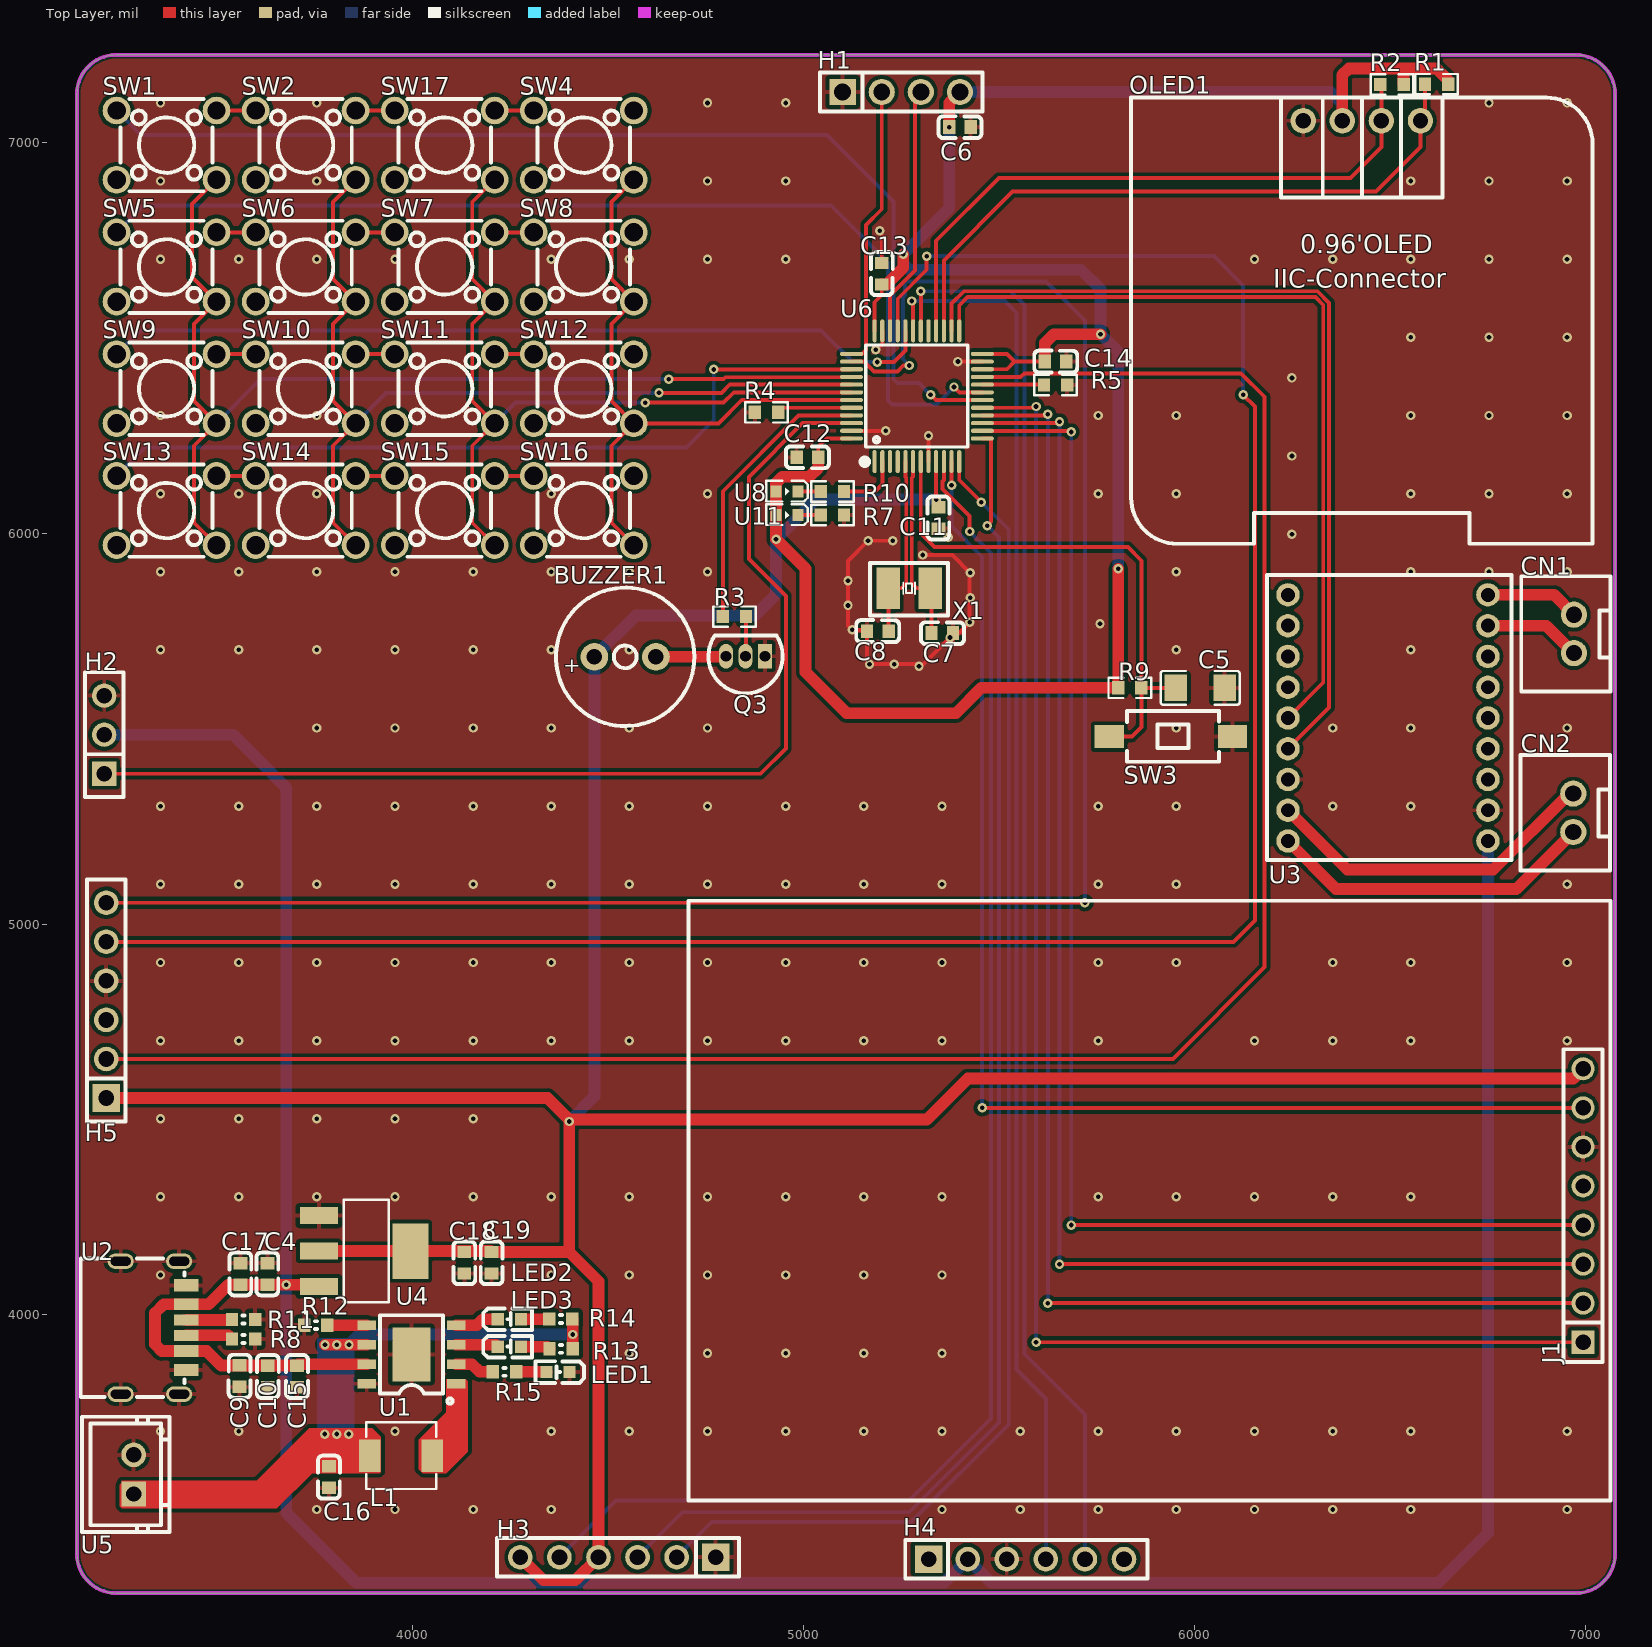
[diagram p0: Top Layer view]
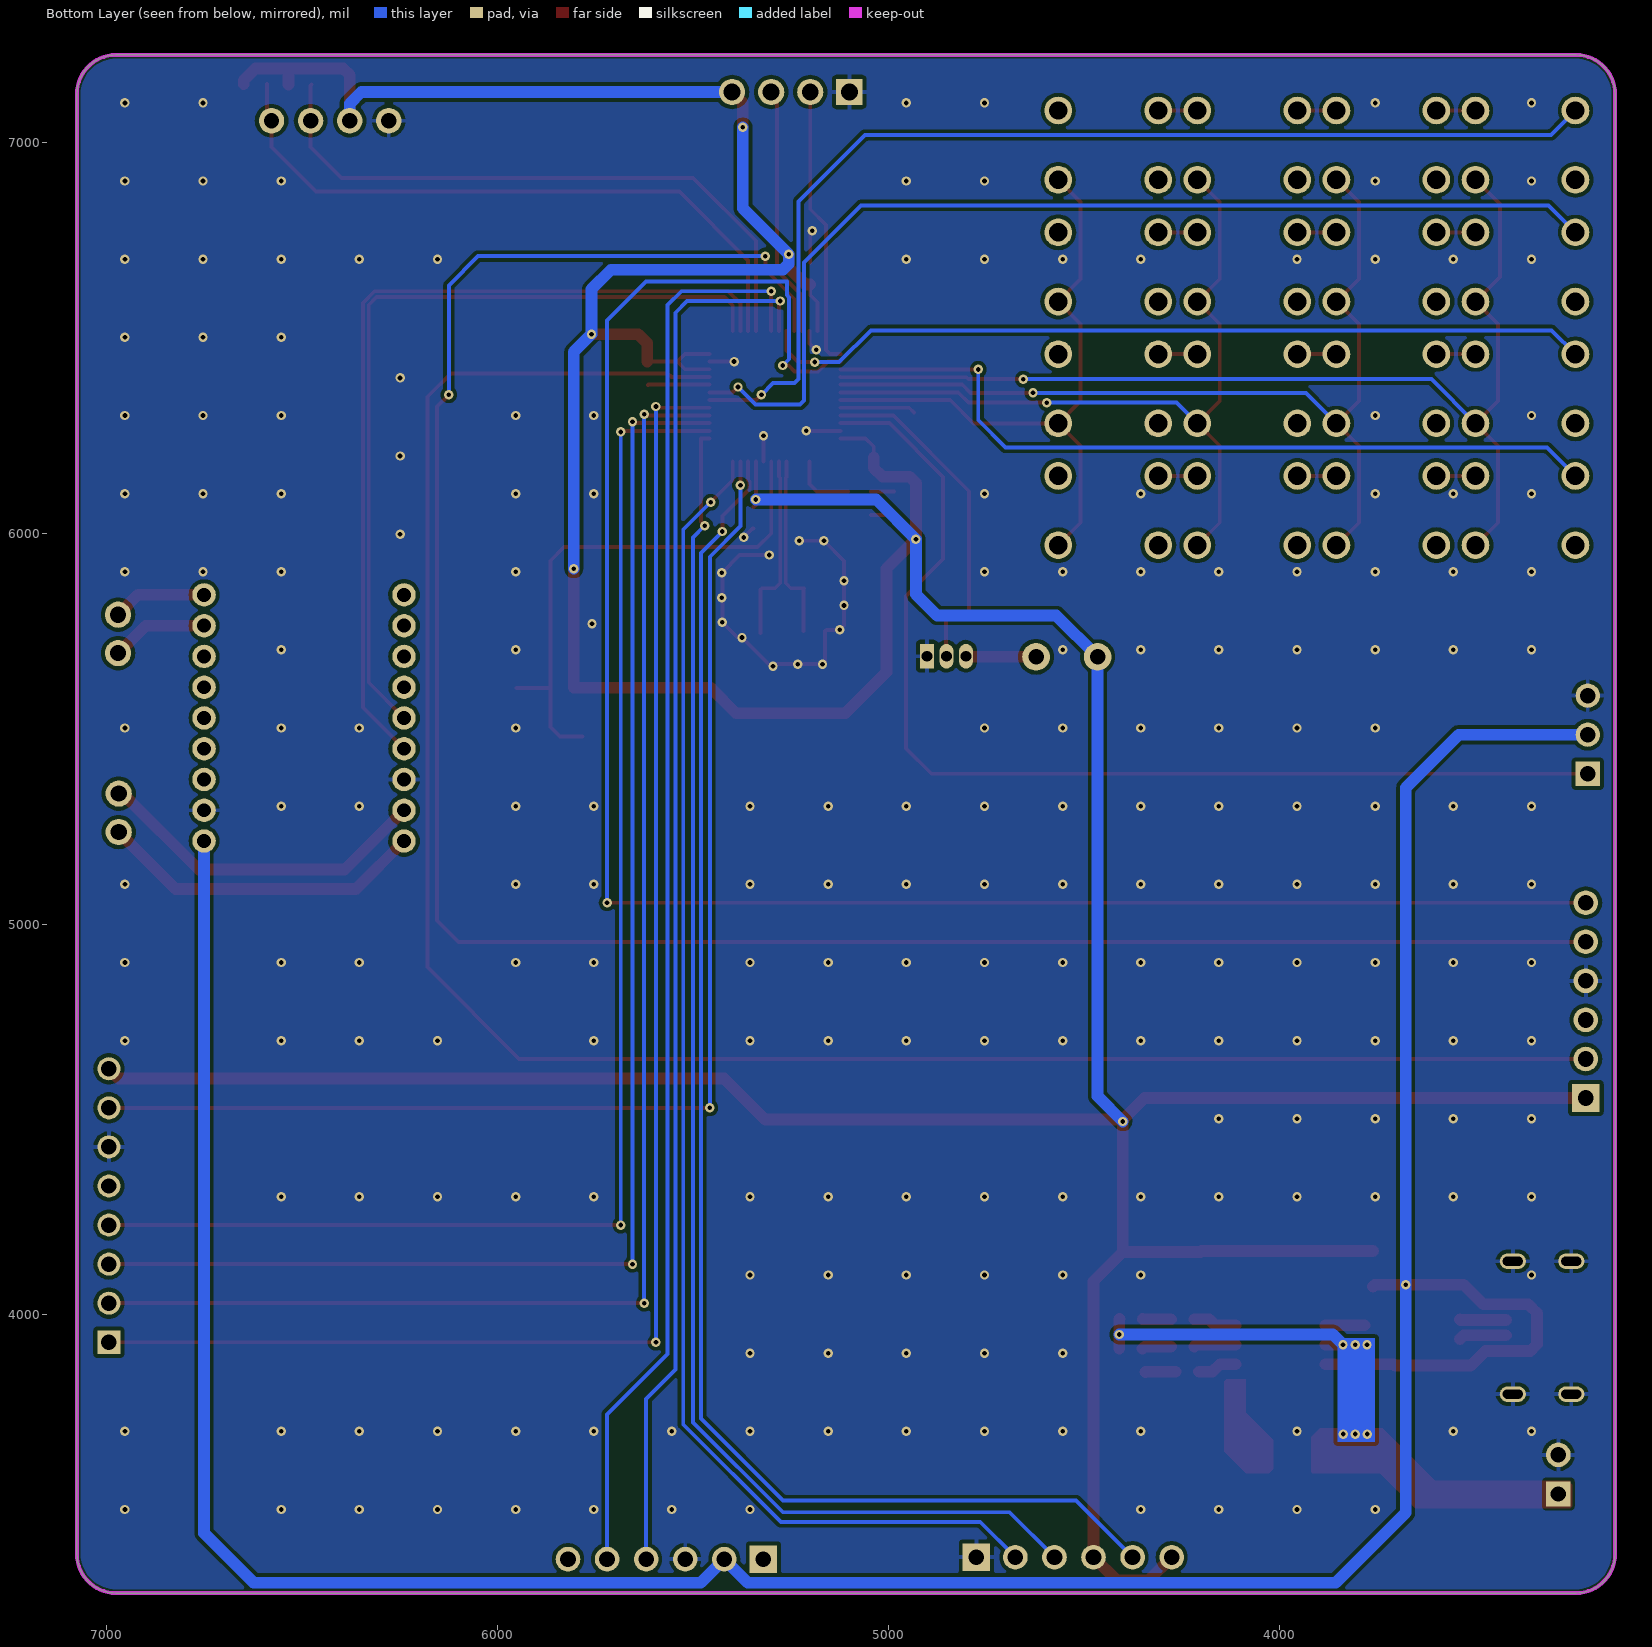
[diagram p1: Bottom Layer view, seen from below]
# Altium PCB MISC52129.pcbdoc
Units mil, origin at the board's own origin, x right, y up, seen from the top; angles counter-clockwise.
Board outline 3937.01 x 3937.01 mil, 2 copper layers (Top Layer, Bottom Layer), stack 62.206 mil thick; 71 components, 74 nets, 277 pads, 263 vias.

## Layer stack, top to bottom
Top Solder Mask Layer: solder mask 0.394, Dk 3.3
Top Layer: signal copper 1.379
Dielectric1: surface 59.449, FR4, Dk 4.5
Bottom Layer: signal copper 1.378
Bottom Solder Mask Layer: solder mask 0.394, Dk 3.3

## Board outline
3240,7225 ccw(c3240,7125) 3140,7125 3140,3387.99 ccw(c3240,3387.99) 3240,3287.99 6977.01,3287.99 ccw(c6977.01,3387.99) 7077.01,3387.99 7077.01,7125 ccw(c6977.01,7125) 6977.01,7225

## Design rules (kind name [scope] priority, off if disabled: settings)
BoardOutlineClearance copperThickness2oz_1 [All] p2 off: genericclearance=7.99 ignorepadtopadclearanceinfootprint=FALSE except(0: Arc-SplitContinuation Track-SplitContinuation SMDPad-SplitContinuation THPad-SplitContinuation Via-SplitContinuation Fill-SplitContinuation Region-SplitContinuation Poly-SplitContinuation Text-SplitContinuation Hole-SplitContinuation; 5.98: Arc-CutoutEdge Track-CutoutEdge SMDPad-CutoutEdge THPad-CutoutEdge Via-CutoutEdge Text-CutoutEdge; 6.9: Hole-OutlineEdge Hole-CutoutEdge; 10: Poly-OutlineEdge Poly-CutoutEdge; 11.81: Arc-OutlineEdge Track-OutlineEdge SMDPad-OutlineEdge THPad-OutlineEdge Via-OutlineEdge Fill-OutlineEdge Region-OutlineEdge Text-OutlineEdge Fill-CutoutEdge Region-CutoutEdge)
BoardOutlineClearance Plane_innerPlane_1 [All] p4 off: genericclearance=4.02 ignorepadtopadclearanceinfootprint=FALSE except(0: Arc-SplitContinuation Track-SplitContinuation SMDPad-SplitContinuation THPad-SplitContinuation Via-SplitContinuation Fill-SplitContinuation Region-SplitContinuation Poly-SplitContinuation Text-SplitContinuation Hole-SplitContinuation; 5.98: Arc-CutoutEdge Track-CutoutEdge SMDPad-CutoutEdge THPad-CutoutEdge Via-CutoutEdge Text-CutoutEdge; 6.9: Hole-OutlineEdge Hole-CutoutEdge; 10: Poly-OutlineEdge Poly-CutoutEdge; 11.81: Arc-OutlineEdge Track-OutlineEdge SMDPad-OutlineEdge THPad-OutlineEdge Via-OutlineEdge Fill-OutlineEdge Region-OutlineEdge Text-OutlineEdge Fill-CutoutEdge Region-CutoutEdge)
BoardOutlineClearance Copper_copperRegion_1 [All] p6 off: genericclearance=4.02 ignorepadtopadclearanceinfootprint=FALSE except(0: Arc-SplitContinuation Track-SplitContinuation SMDPad-SplitContinuation THPad-SplitContinuation Via-SplitContinuation Fill-SplitContinuation Region-SplitContinuation Poly-SplitContinuation Text-SplitContinuation Hole-SplitContinuation; 5.98: Arc-CutoutEdge Track-CutoutEdge SMDPad-CutoutEdge THPad-CutoutEdge Via-CutoutEdge Text-CutoutEdge; 6.9: Hole-OutlineEdge Hole-CutoutEdge; 10: Poly-OutlineEdge Poly-CutoutEdge; 11.81: Arc-OutlineEdge Track-OutlineEdge SMDPad-OutlineEdge THPad-OutlineEdge Via-OutlineEdge Fill-OutlineEdge Region-OutlineEdge Text-OutlineEdge Fill-CutoutEdge Region-CutoutEdge)
BoardOutlineClearance copperThickness1oz_1 [All] p8: genericclearance=4.02 ignorepadtopadclearanceinfootprint=FALSE except(0: Arc-SplitContinuation Track-SplitContinuation SMDPad-SplitContinuation THPad-SplitContinuation Via-SplitContinuation Fill-SplitContinuation Region-SplitContinuation Poly-SplitContinuation Text-SplitContinuation Hole-SplitContinuation; 5.98: Arc-CutoutEdge Track-CutoutEdge SMDPad-CutoutEdge THPad-CutoutEdge Via-CutoutEdge Text-CutoutEdge; 6.9: Hole-OutlineEdge Hole-CutoutEdge; 10: Poly-OutlineEdge Poly-CutoutEdge; 11.81: Arc-OutlineEdge Track-OutlineEdge SMDPad-OutlineEdge THPad-OutlineEdge Via-OutlineEdge Fill-OutlineEdge Region-OutlineEdge Text-OutlineEdge Fill-CutoutEdge Region-CutoutEdge)
Clearance copperThickness2oz [All] p1 off: gap=7.99 ignorepadtopadclearanceinfootprint=FALSE except(5.98: SMDPad-Track SMDPad-SMDPad THPad-Track SMDPad-THPad THPad-THPad Track-Via SMDPad-Via THPad-Via Via-Via Fill-SMDPad Region-SMDPad Fill-THPad Region-THPad Fill-Via Region-Via Fill-Fill Fill-Region Region-Region Arc-Track Arc-SMDPad Arc-THPad Arc-Via Fill-Arc Region-Arc Arc-Arc Text-Track SMDPad-Text Text-THPad Text-Via Fill-Text Region-Text Arc-Text Text-Text; 6.9: Hole-Track Hole-SMDPad Hole-THPad Hole-Via Fill-Hole Region-Hole Hole-Arc Hole-Text; 10: Poly-Track Poly-SMDPad Poly-THPad Poly-Via Poly-Fill Poly-Region Poly-Poly Poly-Arc Poly-Text Poly-Hole; 11.81: Fill-Track Region-Track)
Clearance Plane_innerPlane [All] p3 off: gap=4.02 ignorepadtopadclearanceinfootprint=FALSE except(5.98: SMDPad-Track SMDPad-SMDPad THPad-Track SMDPad-THPad THPad-THPad Track-Via SMDPad-Via THPad-Via Via-Via Fill-SMDPad Region-SMDPad Fill-THPad Region-THPad Fill-Via Region-Via Fill-Fill Fill-Region Region-Region Arc-Track Arc-SMDPad Arc-THPad Arc-Via Fill-Arc Region-Arc Arc-Arc Text-Track SMDPad-Text Text-THPad Text-Via Fill-Text Region-Text Arc-Text Text-Text; 6.9: Hole-Track Hole-SMDPad Hole-THPad Hole-Via Fill-Hole Region-Hole Hole-Arc Hole-Text; 10: Poly-Track Poly-SMDPad Poly-THPad Poly-Via Poly-Fill Poly-Region Poly-Poly Poly-Arc Poly-Text Poly-Hole; 11.81: Fill-Track Region-Track)
Clearance Copper_copperRegion [All] p5 off: gap=4.02 ignorepadtopadclearanceinfootprint=FALSE except(5.98: SMDPad-Track SMDPad-SMDPad THPad-Track SMDPad-THPad THPad-THPad Track-Via SMDPad-Via THPad-Via Via-Via Fill-SMDPad Region-SMDPad Fill-THPad Region-THPad Fill-Via Region-Via Fill-Fill Fill-Region Region-Region Arc-Track Arc-SMDPad Arc-THPad Arc-Via Fill-Arc Region-Arc Arc-Arc Text-Track SMDPad-Text Text-THPad Text-Via Fill-Text Region-Text Arc-Text Text-Text; 6.9: Hole-Track Hole-SMDPad Hole-THPad Hole-Via Fill-Hole Region-Hole Hole-Arc Hole-Text; 10: Poly-Track Poly-SMDPad Poly-THPad Poly-Via Poly-Fill Poly-Region Poly-Poly Poly-Arc Poly-Text Poly-Hole; 11.81: Fill-Track Region-Track)
Clearance copperThickness1oz [All] p7: gap=4.02 ignorepadtopadclearanceinfootprint=FALSE except(5.98: SMDPad-Track SMDPad-SMDPad THPad-Track SMDPad-THPad THPad-THPad Track-Via SMDPad-Via THPad-Via Via-Via Fill-SMDPad Region-SMDPad Fill-THPad Region-THPad Fill-Via Region-Via Fill-Fill Fill-Region Region-Region Arc-Track Arc-SMDPad Arc-THPad Arc-Via Fill-Arc Region-Arc Arc-Arc Text-Track SMDPad-Text Text-THPad Text-Via Fill-Text Region-Text Arc-Text Text-Text; 6.9: Hole-Track Hole-SMDPad Hole-THPad Hole-Via Fill-Hole Region-Hole Hole-Arc Hole-Text; 10: Poly-Track Poly-SMDPad Poly-THPad Poly-Via Poly-Fill Poly-Region Poly-Poly Poly-Arc Poly-Text Poly-Hole; 11.81: Fill-Track Region-Track)
DiffPairsRouting differentialPair [All] p1: maxlimit=6 minlimit=6 mostfreqgap=6 toplayer_minwidth=5 toplayer_prefwidth=10 toplayer_maxwidth=100 toplayer_mingap=6 toplayer_prefgap=6 toplayer_maxgap=6 bottomlayer_minwidth=5 bottomlayer_prefwidth=10 bottomlayer_maxwidth=100 bottomlayer_mingap=6 bottomlayer_prefgap=6 bottomlayer_maxgap=6 maxuncoupledlength=10
HoleToHoleClearance otherClearance [All] p1: gap=11.81 allowstackedmicrovias=TRUE
Length netLength [All] p1: minlimit=0 maxlimit=0
PasteMaskExpansion pasteMaskExpansion [All] p1: expansion=0
PlaneConnect innerPlane [All] p1: planeconnectstyle=Relief reliefexpansion=20 reliefentries=4 reliefconductorwidth=10 reliefairgap=10
PolygonConnect copperRegion [All] p1: connectstyle=Relief reliefconductorwidth=10 reliefentries=4 polygonreliefangle="90 Angle" airgapwidth=10 via.connectstyle=Relief via.reliefconductorwidth=10 via.reliefentries=4 via.polygonreliefangle="90 Angle" via.airgapwidth=10
RoutingVias viaSize [All] p1: holewidth=12.01 width=24.02 viastyle="Through Hole" minholewidth=11.81 minwidth=19.68 maxholewidth=248.03 maxwidth=393.7
SolderMaskExpansion solderMaskExpansion [IsVia] p1: expansion=-1000 istentingtop=TRUE
SolderMaskExpansion solderMaskExpansion [All] p2: expansion=2 istentingtop=FALSE
Width copperThickness2oz_2 [All] p1 off: maxlimit=100 minlimit=8 preferedwidth=10
Width copperThickness1oz_2 [All] p2: maxlimit=100 minlimit=5 preferedwidth=10

## Components (designator, comment, footprint, x,y, rotation, side; value= is the part's Value field where it differs from the comment)
BUZZER1 "2.7kHz" BUZ-TH_BD9.0-P4.00-D0.6-FD 4543.28,5684.32 r0 top
C4 "10uF" C0603 3627.51,4104.85 r270 top
C5 "100uF" C1206 6015,5605 r180 top
C6 "100nF" C0603 5400,7040 r180 top
C7 "20pF" C0603 5355,5745 r180 top
C8 "20pF" C0603 5190,5750 r0 top
C9 "22uF" C0603 3556.59,3843.41 r90 top
C10 "22uF" C0603 3628.64,3842.73 r90 top
C11 "100nF" C0603 5345,6040 r90 top
C12 "100nF" C0603 5010,6195 r0 top
C13 "100nF" C0603 5200,6665 r270 top
C14 "100nF" C0603 5645,6440 r180 top
C15 "22uF" C0603 3703.38,3842.73 r90 top
C16 "22uF" C0603 3785,3585 r90 top
C17 "100nF" C0603 3558.38,4104.85 r270 top
C18 "10uF" C0603 4131.59,4133.41 r90 top
C19 "100nF" C0603 4201.59,4133.41 r90 top
CN1 "XH2.54*2P_直插" CONN-TH_2P-P2.50-XH2.54-2P 6971.54,5742.95 r270 top
CN2 "XH2.54*2P_直插" CONN-TH_2P-P2.50-XH2.54-2P 6970,5285 r270 top
H1 "" HDR-TH_4P-P2.54-V-F 5250,7130 r0 top
H2 "" HDR-TH_3P-P2.54-V-F 3210,5485 r90 top
H3 "" HDR-TH_6P-P2.54-V-F 4525,3380 r180 top
H4 "" HDR-TH_6P-P2.54-V-F 5570,3375 r0 top
H5 "" HDR-TH_6P-P2.54-V-F 3215,4805 r90 top
J1 "" HDR-TH_8P-P2.54-V-M 6995,4280 r90 top
L1 "2.2uH" IND-SMD_L4.4-W4.2 3970,3640 r180 top
LED1 "电池" LED0603_L1.6-W0.8-RD_BLUE 4371.39,3853.75 r180 top
LED2 "放电" LED0603_L1.6-W0.8-RD_BLUE 4247.02,3988.81 r0 top
LED3 "充电" LED0603_L1.6-W0.8-RD_BLUE 4247.02,3918.81 r0 top
OLED1 "" 0.96OLED_4P 6428.8,7056.43 r0 top
Q3 "" S8050_TO_92 4851.43,5685.89 r180 top
R1 "5.1K" R0603 6620,7150 r0 top
R2 "5.1K" R0603 6505.98,7149.32 r0 top
R3 "1K" R0603 4822.85,5787.32 r180 top
R4 "10kΩ" R0603 4905,6310 r0 top
R5 "10kΩ" R0603 5645,6380 r180 top
R7 "510Ω" R0603 5073.8,6047.22 r0 top
R8 "5.1K" R0603-NSK 3566.59,3938.41 r180 top
R9 "1kΩ" R0603 5835,5605 r180 top
R10 "510Ω" R0603 5073.8,6107.52 r0 top
R11 "5.1K" R0603-NSK 3566.59,3988.41 r180 top
R12 "56K" R0603-NSK 3751.59,3973.91 r180 top
R13 "5.1K" R0603-NSK 4379.2,3913.13 r180 top
R14 "5.1K" R0603-NSK 4378.67,3989.49 r180 top
R15 "5.1K" R0603-NSK 4234.52,3854.37 r180 top
SW1 "KH-6X6X6H-TJ" SW-TH_4P-L6.0-W6.0-P4.50-LS6.5 3369.4,6994.04 r0 top
SW2 "KH-6X6X6H-TJ" SW-TH_4P-L6.0-W6.0-P4.50-LS6.5 3725.37,6994.04 r0 top
SW3 "TS-1101-C-W" SW-SMD_L6.0-W3.3-LS8.0 5940,5480 r180 top
SW4 "KH-6X6X6H-TJ" SW-TH_4P-L6.0-W6.0-P4.50-LS6.5 4437.3,6994.04 r0 top
SW5 "KH-6X6X6H-TJ" SW-TH_4P-L6.0-W6.0-P4.50-LS6.5 3369.4,6682.26 r0 top
SW6 "KH-6X6X6H-TJ" SW-TH_4P-L6.0-W6.0-P4.50-LS6.5 3725.37,6682.26 r0 top
SW7 "KH-6X6X6H-TJ" SW-TH_4P-L6.0-W6.0-P4.50-LS6.5 4081.33,6682.26 r0 top
SW8 "KH-6X6X6H-TJ" SW-TH_4P-L6.0-W6.0-P4.50-LS6.5 4437.3,6682.26 r0 top
SW9 "KH-6X6X6H-TJ" SW-TH_4P-L6.0-W6.0-P4.50-LS6.5 3369.4,6370.49 r0 top
SW10 "KH-6X6X6H-TJ" SW-TH_4P-L6.0-W6.0-P4.50-LS6.5 3725.37,6370.49 r0 top
SW11 "KH-6X6X6H-TJ" SW-TH_4P-L6.0-W6.0-P4.50-LS6.5 4081.33,6370.49 r0 top
SW12 "KH-6X6X6H-TJ" SW-TH_4P-L6.0-W6.0-P4.50-LS6.5 4437.3,6370.49 r0 top
SW13 "KH-6X6X6H-TJ" SW-TH_4P-L6.0-W6.0-P4.50-LS6.5 3369.4,6058.72 r0 top
SW14 "KH-6X6X6H-TJ" SW-TH_4P-L6.0-W6.0-P4.50-LS6.5 3725.37,6058.72 r0 top
SW15 "KH-6X6X6H-TJ" SW-TH_4P-L6.0-W6.0-P4.50-LS6.5 4081.33,6058.72 r0 top
SW16 "KH-6X6X6H-TJ" SW-TH_4P-L6.0-W6.0-P4.50-LS6.5 4437.3,6058.72 r0 top
SW17 "KH-6X6X6H-TJ" SW-TH_4P-L6.0-W6.0-P4.50-LS6.5 4081.33,6994.04 r0 top
U1 "ETA9742" ESOP-8_L4.9-W3.9-P1.27-LS6.0-BL-EP 3996.39,3898.81 r90 top
U2 "YTC-TC6-268" TYPE-C-SMD_YIYUAN_YTC-TC6-268 3335.87,3967.32 r270 top
U3 "CON2.0MM-PAD-18" CONN-TH_18P-P2.00_C9900078766 6751.54,5527.95 r90 top
U4 "AMS1117-3.3" SOT-223-3_L6.5-W3.4-P2.30-LS7.0-BR 3876.59,4163.41 r180 top
U5 "_x001F_XH2.54-2P" CONN-TH_2P-P2.54-V 3285.24,3591.72 r90 top
U6 "STM32F103C8T6" LQFP-48_L7.0-W7.0-P0.50-LS9.0-BL 5290.06,6351.43 r0 top
U8 "42-51/GHC-YW2X2K/3T" LED-SMD_L1.6-W0.8-FD_GREEN-1 4957.67,6107.52 r0 top
U11 "42-51/GHC-YW2X2K/3T" LED-SMD_L1.6-W0.8-FD_GREEN-1 4957.67,6047.22 r0 top
X1 "8MHz" CRYSTAL-SMD_L3.2-W2.5_3225-8MHZ 5270,5860 r180 top

## Footprints (in the part's own frame and the unit in brackets; to place one, negate y for a bottom-side part, rotate by r counter-clockwise, add the part's x,y. Pads: shape width x height; smd on the part's side, far side on the other; paste and mask are expansions set on the pad)
0.96OLED_4P [mm]
  round 1.65 hole 1 copper offset 0,0: 1(-3.81,-0.001) 2(-1.27,0.002) 3(1.27,0.002) 4(3.81,0.002)
  silkscreen extent -15,-27.5 15,1.5
BUZ-TH_BD9.0-P4.00-D0.6-FD [mm]
  round 1.8 hole 1: 1(-2,0) 2(2,0)
  silkscreen extent -4.5,-4.5 4.5,4.5
C0603 [mm]
  rect 0.8x0.9 smd: 1(-0.7,0) 2(0.7,0)
  silkscreen extent -1.39,-0.71 1.39,0.71
C1206 [mm]
  rect 1.485x1.728 smd paste-100 mask+0.051: 1(-1.593,0) 2(1.593,0)
  silkscreen extent -2.56,-1.09 2.56,1.09
CONN-TH_2P-P2.50-XH2.54-2P [mm]
  round 1.7 hole 1.05 paste+0 mask+0.05: 1(1.25,0) 2(-1.25,0)
  silkscreen extent -3.75,-3.42 3.75,2.37
CONN-TH_2P-P2.54-V [mm]
  rect 1.6x1.6 hole 1: 1(-1.27,0)
  round 1.6 hole 1: 2(1.27,0)
  silkscreen extent -3.75,-2.34 3.75,3.36
CONN-TH_18P-P2.00_C9900078766 [mil]
  round 60 hole 35.43 paste+0 mask+1.97: 1(-314.96,0.01) 2(-314.96,511.81) 3(-236.22,0.01) 4(-236.22,511.81) 5(-157.48,0.01) 6(-157.48,511.81) 9(0,0) 10(0,511.81) 11(78.74,0) 12(78.74,511.81) 13(157.48,0) 14(157.48,511.81) 15(236.22,0) 16(236.22,511.81) 17(314.96,0) 18(314.96,511.81)
  round 60 hole 35.43 copper offset -0.01,0 paste+0 mask+1.97: 7(-78.72,0.01) 8(-78.72,511.81)
  silkscreen extent -363,-60 365,565
CRYSTAL-SMD_L3.2-W2.5_3225-8MHZ [mil]
  rect 60x106.3 smd paste+0 mask+1.97: 1(-53.62,0) 2(53.62,0)
  silkscreen extent -100,-65 100,70
ESOP-8_L4.9-W3.9-P1.27-LS6.0-BL-EP [mm]
  rect 0.6x1.2 smd paste+0 mask+0.051: 1(-1.905,-2.908) 2(-0.635,-2.908) 3(0.635,-2.908) 4(1.905,-2.908) 5(1.905,2.908) 6(0.635,2.908) 7(-0.635,2.908) 8(-1.905,2.908)
  rect 3.5x2.5 smd paste+0 mask+0.051: 9(0,0)
  silkscreen extent -3.2,-2.67 2.55,2.05
HDR-TH_3P-P2.54-V-F [mil]
  rect 62x62 hole 40.16: 1(-100,0)
  round 62 hole 40.16: 2(0,0) 3(100,0)
  silkscreen extent -160,-49 160,49
HDR-TH_4P-P2.54-V-F [mm]
  rect 1.7x1.7 hole 1.1: 1(-3.81,0)
  round 1.7 hole 1.1: 2(-1.27,0) 3(1.27,0) 4(3.81,0)
  silkscreen extent -5.29,-1.27 5.29,1.27
HDR-TH_6P-P2.54-V-F [mm]
  rect 1.8x1.8 hole 1.02: 1(-6.35,0)
  round 1.6 hole 1.02: 2(-3.81,0) 3(-1.27,0) 4(1.27,0) 5(3.81,0) 6(6.35,0)
  silkscreen extent -7.87,-1.25 7.87,1.25
HDR-TH_8P-P2.54-V-M [mm]
  rect 1.5x1.5 hole 1: 1(-8.89,0)
  round 1.5 hole 1: 2(-6.35,0) 3(-3.81,0) 4(-1.27,0) 5(1.27,0) 6(3.81,0) 7(6.35,0) 8(8.89,0)
  silkscreen extent -10.16,-1.27 10.16,1.27
IND-SMD_L4.4-W4.2 [mm]
  rect 1.4x2.12 smd paste+0 mask+0.051: 1(2.028,0) 2(-2.028,0)
  silkscreen extent -2.28,-2.18 2.28,2.18
LED0603_L1.6-W0.8-RD_BLUE [mm]
  rect 0.8x0.8 smd: 1(-0.75,0) 2(0.75,0)
  silkscreen extent -1.7,-0.7 1.47,0.7
LED-SMD_L1.6-W0.8-FD_GREEN-1 [mm]
  rect 0.7x0.8 smd: 1(-0.715,0) 2(0.715,0)
  silkscreen extent -1.35,-0.65 1.35,0.7
LQFP-48_L7.0-W7.0-P0.50-LS9.0-BL [mm]
  oval 0.27x1.5 smd paste+0 mask+0.05: 1(-2.75,-4.25) 2(-2.25,-4.25) 3(-1.75,-4.25) 4(-1.25,-4.25) 5(-0.75,-4.25) 6(-0.25,-4.25) 7(0.25,-4.25) 8(0.75,-4.25) 9(1.25,-4.25) 10(1.75,-4.25) 11(2.25,-4.25) 12(2.75,-4.25) 25(2.75,4.25) 26(2.25,4.25) 27(1.75,4.25) 28(1.25,4.25) 29(0.75,4.25) 30(0.25,4.25) 31(-0.25,4.25) 32(-0.75,4.25) 33(-1.25,4.25) 34(-1.75,4.25) 35(-2.25,4.25) 36(-2.75,4.25)
  oval 1.5x0.27 smd paste+0 mask+0.05: 13(4.25,-2.75) 14(4.25,-2.25) 15(4.25,-1.75) 16(4.25,-1.25) 17(4.25,-0.75) 18(4.25,-0.25) 19(4.25,0.25) 20(4.25,0.75) 21(4.25,1.25) 22(4.25,1.75) 23(4.25,2.25) 24(4.25,2.75) 37(-4.25,2.75) 38(-4.25,2.25) 39(-4.25,1.75) 40(-4.25,1.25) 41(-4.25,0.75) 42(-4.25,0.25) 43(-4.25,-0.25) 44(-4.25,-0.75) 45(-4.25,-1.25) 46(-4.25,-1.75) 47(-4.25,-2.25) 48(-4.25,-2.75)
  silkscreen extent -3.59,-4.46 3.3,3.34
R0603 [mil]
  rect 31.75x34.02 smd paste-3937.01 mask+2: 1(-29.66,0) 2(29.66,0)
  silkscreen extent -55,-26 55,26
R0603-NSK [mil]
  rect 31.75x34.02 smd paste-3937.01 mask+2: 1(-29.65,0) 2(29.66,0)
  silkscreen extent -3,-10 3,10
S8050_TO_92 [mil]
  rect 35.4x63 hole 27.6 paste+0 mask+2: 1(-50,0)
  oval 35.4x63 hole 27.6 paste+0 mask+2: 2(0,0) 3(50,0)
  silkscreen extent -95,-53 95,95
SOT-223-3_L6.5-W3.4-P2.30-LS7.0-BR [mm]
  rect 2.5x1.1 smd: 1(2.97,-2.3) 2(2.97,0) 3(2.97,2.3)
  rect 2.34x3.6 smd: 4(-2.97,0)
  silkscreen extent -1.57,-3.33 1.37,3.33
SW-SMD_L6.0-W3.3-LS8.0 [mm]
  rect 1.9x1.5 smd: 1(-4,0) 2(4,0)
  silkscreen extent -3.14,-1.67 2.86,1.63
SW-TH_4P-L6.0-W6.0-P4.50-LS6.5 [mm]
  round 1.8 hole 1.2: 1(-3.25,2.25) 2(3.25,2.25) 3(-3.25,-2.25) 4(3.25,-2.25)
  silkscreen extent -3,-3 3,3
TYPE-C-SMD_YIYUAN_YTC-TC6-268 [mm]
  oval 1x1.7 hole 0.6 slot 1.3 at 90 deg paste+0 mask+0.05: 1(-4.32,1.676) 2(4.32,1.676) 3(4.32,-2.125) 4(-4.32,-2.125)
  rect 0.7x1.6 smd paste-100 mask+0.05: A5(-0.5,2.125) B5(0.5,2.125)
  rect 0.76x1.6 smd paste-100 mask+0.05: A9(1.52,2.125) B9(-1.52,2.125)
  rect 0.8x1.6 smd paste-100 mask+0.05: A12(2.75,2.125) B12(-2.75,2.125)
  silkscreen extent -4.5,-4.72 4.5,2.03

## Via types
v1: diameter 24.02, hole 12, Top Layer to Bottom Layer, 263 vias

## Nets (pads, with @x,y where several pads share a name; then routed paths per layer and width w, separated by ;. In a path a pad name is that pad's centre, name@x,y a point inside that pad or via, vN(x,y) a via of type N, cw(c..) or ccw(c..) an arc to the next point about the centre after c; other vN are vias at no path point)
$1N1877: BUZZER1.2 Q3.3 | length 180.1
  Top Layer w30: BUZZER1.2 4799.86,5684.32 Q3.3
$1N2018: Q3.2 R3.1 | length 101.9
  Top Layer w10: Q3.2 4852.51,5686.98 R3.1
$1N5108: R7.1 U11.2 | length 58.3
  Top Layer w10: U11.2 R7.1
$1N5109: R10.1 U8.2 | length 58.3
  Top Layer w10: U8.2 R10.1
$1N5277: SW9.2 SW10.1 | length 100.1
  Top Layer w10: SW9.2 SW10.1
$1N5278: SW13.2 SW14.1 | length 100.1
  Top Layer w10: SW13.2 SW14.1
$1N5279: SW15.2 SW16.1 | length 100.1
  Top Layer w10: SW15.2 SW16.1@4309.35,6147.3
$1N5280: SW14.2 SW15.1 | length 100.1
  Top Layer w10: SW14.2 SW15.1
$1N5281: SW11.2 SW12.1 | length 100.1
  Top Layer w10: SW11.2 SW12.1@4309.35,6459.07
$1N5282: SW10.2 SW11.1 | length 100.1
  Top Layer w10: SW10.2 SW11.1
$1N5283: SW7.2 SW8.1 | length 100.1
  Top Layer w10: SW7.2 SW8.1@4309.35,6770.84
$1N5284: SW5.2 SW6.1 | length 100.1
  Top Layer w10: SW5.2 SW6.1
$1N5285: SW6.2 SW7.1 | length 100.1
  Top Layer w10: SW6.2 SW7.1
$1N5286: SW1.2 SW2.1 | length 100.1
  Top Layer w10: SW1.2 SW2.1
$1N5287: SW2.2 SW17.1 | length 100.1
  Top Layer w10: SW2.2 SW17.1
$1N5288: SW4.1 SW17.2 | length 100.1
  Top Layer w10: SW17.2 SW4.1@4309.35,7082.62
$1N5308: LED3.2 R13.2 | length 75.3
  Top Layer w30: LED3.2 4343.87,3918.81 R13.2
$1N5310: LED1.2 R15.1 | length 77.9
  Top Layer w30: R15.1 4341.24,3854.37 LED1.2
$1N5311: LED2.2 R14.2 | length 72.8
  Top Layer w30: LED2.2 4348.33,3988.81 R14.2
$1N5312: LED2.1 U1.4 | length 112.8
  Top Layer w30: U1.4 4163.81,3973.81 4178.81,3988.81 LED2.1
$1N5313: R8.2 U2.B5 | length 121.2
  Top Layer w30: U2.B5 3527.72,3947.63 R8.2
$1N5314: R11.2 U2.A5 | length 118
  Top Layer w30: U2.A5 3535.52,3987 R11.2
$1N5317: LED3.1 U1.3 | length 108.7
  Top Layer w30: U1.3 4212.49,3923.81 LED3.1
$1N5319: R15.2 U1.2 | length 102
  Top Layer w30: U1.2 4151.19,3873.81 4170.63,3854.37 R15.2
$1N5320: R12.1 U1.5 | length 100.7
  Top Layer w30: R12.1 3881.79,3973.91 U1.5
$1N5322: L1.2 U1.1
+5V: C4.2 C9.2 C10.2 C15.2 C17.2 H2.2 H4.2 U1.7 U2.A9 U2.B9 U3.1 U4.3 | length 8498.4
  Top Layer w30: U4.3 3755.24,4077.29 v1(3676,4077.29) C4.2 C17.2 3527.29,4077.29 3477.16,4027.16 U2.B9 3362.16,4027.16 3340,4005 3340,3925 3357.53,3907.47 U2.A9 3472.53,3907.47 3509.71,3870.29 C10.2 C15.2 3706.9,3873.81 U1.7
  Bottom Layer w30: H2.2 3540,5485 3676,5349 v1(3676,4077.29) 3676,3494 3855.2,3314.8 5359.8,3314.8 5367.18,3322.18 ccw(c5355.43,3339.57) 5372.82,3327.82 H4.2 5480.2,3314.8 6624.8,3314.8 6751.53,3441.53 U3.1
BAT: C16.2 L1.1 R13.1 R14.1 U1.6 U5.1 | length 766.9
  Top Layer w30: v1(3775,3923.81) v1(3805.38,3923.81) v1(3836.32,3923.81) U1.6 ; R14.1 4408.85,3988.96 v1(4408.85,3950) R13.1
  Bottom Layer w30: v1(3836.32,3923.81) 3862.51,3950 v1(4408.85,3950)
  other v1: 3774.34,3695 3804.73,3695 3835.66,3695
BEEP: R3.2 U6.45 | length 730.8
  Top Layer w10: R3.2 4793.19,6108.19 4987.22,6302.22 U6.45
BOOT0: R4.2 U6.44 | length 193
  Top Layer w10: R4.2 4946.56,6321.9 U6.44
BOOT1: R5.2 U6.20 | length 158.4
  Top Layer w10: U6.20 5614.38,6380.96 R5.2
CLK: H1.2 U6.37 | length 718.1
  Top Layer w10: U6.37 5149.7,6459.7 5160,6470 5160,6790 5200,6830 H1.2
DIO: H1.3 U6.34 | length 643.9
  Top Layer w10: U6.34 5221.16,6609.6 5285,6673.44 5285,7115 H1.3
GND: C4.1 C5.1 C6.1 C7.1 C8.1 C9.1 C10.1 C11.1 C12.1 C13.1 C14.1 C15.1 C16.1 C17.1 C18.1 C19.1 H1.1 H2.3 H3.1 H4.3 H5.4 J1.6 LED1.1 OLED1.1 Q3.1 R4.1 R5.1 R7.2 R8.1 R11.1 R12.2 SW3.1 U1.8 U1.9 U2.1 U2.2 U2.3 U2.4 U2.A12 U2.B12 U3.3 U3.6 U4.1 U5.2 U6.8 U6.23 U6.35 U6.47 | length 1406.2
  Top Layer w10: U6.47 v1(5210,6262.85) ; v1(5185,6470) 5201.48,6486.48 U6.35 ; v1(5195,6775) 5200,6770 C13.1 ; v1(5228.39,5981.38) v1(5165,5981.38) 5113.62,5930 v1(5113.62,5879.29) v1(5113.62,5815.91) 5113.62,5764.28 v1(5124.45,5753.45) 5158.99,5753.45 C8.1 5162.44,5671.95 v1(5168.72,5665.67) v1(5232.1,5665.67) 5290.06,5665.67 v1(5295.27,5660.46) 5301.64,5660.46 v1(5374.81,5733.62) 5385.93,5733.62 v1(5424.84,5772.54) 5424.84,5897.75 v1(5426.38,5899.29) 5380.67,5945 v1(5305,5945) ; U6.8 v1(5319.59,6250) ; C11.1 5347.99,6012.44 v1(5370.44,5989.99) ; v1(5395,6440.01) U6.23
  other v1: 3754.1,3502.09 3954.1,3502.09 4154.1,3502.09 4354.1,3502.09 5354.1,3502.09 5554.1,3502.09 5754.1,3502.09 5954.1,3502.09 6154.1,3502.09 6354.1,3502.09 6554.1,3502.09 6954.1,3502.09 3354.1,3702.09 3554.1,3702.09 3954.1,3702.09 4354.1,3702.09 4554.1,3702.09 4754.1,3702.09 4954.1,3702.09 5154.1,3702.09 5354.1,3702.09 5554.1,3702.09 5754.1,3702.09 5954.1,3702.09 6154.1,3702.09 6354.1,3702.09 6554.1,3702.09 6954.1,3702.09 4554.1,3902.09 4754.1,3902.09 4954.1,3902.09 5154.1,3902.09 5354.1,3902.09 3354.1,4102.09 4354.1,4102.09 4554.1,4102.09 4754.1,4102.09 4954.1,4102.09 5154.1,4102.09 5354.1,4102.09 3354.1,4302.09 3554.1,4302.09 3754.1,4302.09 3954.1,4302.09 4154.1,4302.09 4354.1,4302.09 4554.1,4302.09 4754.1,4302.09 4954.1,4302.09 5154.1,4302.09 5354.1,4302.09 5754.1,4302.09 5954.1,4302.09 6154.1,4302.09 6354.1,4302.09 6554.1,4302.09 3354.1,4502.09 3554.1,4502.09 3754.1,4502.09 3954.1,4502.09 4154.1,4502.09 3354.1,4702.09 3554.1,4702.09 3754.1,4702.09 3954.1,4702.09 4154.1,4702.09 4354.1,4702.09 4554.1,4702.09 4754.1,4702.09 4954.1,4702.09 5154.1,4702.09 5354.1,4702.09 5754.1,4702.09 6154.1,4702.09 6354.1,4702.09 6554.1,4702.09 6954.1,4702.09 3354.1,4902.09 3554.1,4902.09 3754.1,4902.09 3954.1,4902.09 4154.1,4902.09 4354.1,4902.09 4554.1,4902.09 4754.1,4902.09 4954.1,4902.09 5154.1,4902.09 5354.1,4902.09 5754.1,4902.09 5954.1,4902.09 6354.1,4902.09 6554.1,4902.09 6954.1,4902.09 3354.1,5102.09 3554.1,5102.09 3754.1,5102.09 3954.1,5102.09 4154.1,5102.09 4354.1,5102.09 4554.1,5102.09 4754.1,5102.09 4954.1,5102.09 5154.1,5102.09 5354.1,5102.09 5754.1,5102.09 5954.1,5102.09 6954.1,5102.09 3354.1,5302.09 3554.1,5302.09 3754.1,5302.09 3954.1,5302.09 4154.1,5302.09 4354.1,5302.09 4554.1,5302.09 4754.1,5302.09 4954.1,5302.09 5154.1,5302.09 5354.1,5302.09 5754.1,5302.09 5954.1,5302.09 6354.1,5302.09 6554.1,5302.09 3754.1,5502.09 3954.1,5502.09 4154.1,5502.09 4354.1,5502.09 4554.1,5502.09 4754.1,5502.09 5954.1,5502.09 6354.1,5502.09 6554.1,5502.09 6954.1,5502.09 3354.1,5702.09 3554.1,5702.09 3754.1,5702.09 3954.1,5702.09 4154.1,5702.09 4354.1,5702.09 4554.1,5702.09 5954.1,5702.09 6554.1,5702.09 5758.62,5769.1 5426.38,5835.9 3354.1,5902.09 3554.1,5902.09 3754.1,5902.09 3954.1,5902.09 4154.1,5902.09 4354.1,5902.09 4554.1,5902.09 4754.1,5902.09 5954.1,5902.09 6554.1,5902.09 6754.1,5902.09 6954.1,5902.09 6249.78,5998.25 3354.1,6102.09 3554.1,6102.09 3754.1,6102.09 4354.1,6102.09 4754.1,6102.09 5754.1,6102.09 5954.1,6102.09 6554.1,6102.09 6754.1,6102.09 6954.1,6102.09 6249.78,6198.25 3354.1,6302.09 3754.1,6302.09 5754.1,6302.09 5954.1,6302.09 6554.1,6302.09 6754.1,6302.09 6954.1,6302.09 6249.78,6398.25 6554.1,6502.09 6754.1,6502.09 6954.1,6502.09 3354.1,6702.09 3554.1,6702.09 3754.1,6702.09 3954.1,6702.09 4354.1,6702.09 4554.1,6702.09 4754.1,6702.09 4954.1,6702.09 6154.1,6702.09 6354.1,6702.09 6554.1,6702.09 6754.1,6702.09 6954.1,6702.09 3354.1,6902.09 3754.1,6902.09 4754.1,6902.09 4954.1,6902.09 6554.1,6902.09 6754.1,6902.09 6954.1,6902.09 3354.1,7102.09 3754.1,7102.09 4754.1,7102.09 4954.1,7102.09 6754.1,7102.09 6954.1,7102.09
MFR_MISO: J1.4 U6.14 | length 3568.8
  Top Layer w10: U6.14 5682.15,6262.85 v1(5685,6260) ; v1(5685,4230) J1.4
  Bottom Layer w10: v1(5685,4230) v1(5685,6260)
MFR_MOSI: J1.3 U6.15 | length 3694.8
  Top Layer w10: U6.15 5651.69,6282.53 v1(5655,6285.84) ; v1(5655,4130) J1.3
  Bottom Layer w10: v1(5655,4130) v1(5655,6285.84)
MFR_RST: J1.7 U6.11 | length 3224.6
  Top Layer w10: U6.11 5378.64,6123.85 v1(5378.74,6123.74) ; v1(5457.01,4530) J1.7
  Bottom Layer w10: v1(5378.74,6123.74) 5378.74,6018.74 5457.01,5940.48 v1(5457.01,4530)
MFR_SCK: J1.2 U6.16 | length 3814.5
  Top Layer w10: U6.16 5621.7,6302.22 v1(5625,6305.52) ; v1(5625,4030) J1.2
  Bottom Layer w10: v1(5625,4030) v1(5625,6305.52)
MFR_SDA: J1.1 U6.17 | length 3934.2
  Top Layer w10: U6.17 5591.69,6321.9 v1(5595,6325.21) ; v1(5595,3930) J1.1
  Bottom Layer w10: v1(5595,3930) v1(5595,6325.21)
MIC+: CN1.1 U3.15 | length 249.2
  Top Layer w30: U3.15 6901.1,5764.17 CN1.1
MIC-: CN1.2 U3.17 | length 241
  Top Layer w30: U3.17 6920.79,5842.91 CN1.2
OLED_SCL: OLED1.3 R2.1 U6.28 | length 1630.8
  Top Layer w10: U6.28 5339.27,6749.27 5500,6910 6400,6910 6478.8,6988.8 OLED1.3 6478.8,7146.84 R2.1
OLED_SDA: OLED1.4 R1.1 U6.27 | length 1686.1
  Top Layer w10: U6.27 5358.96,6698.96 5535,6875 6465,6875 6578.8,6988.8 OLED1.4 6590.34,7068.02 R1.1
OSC32-IN: U6.3
OSC32-OUT: U6.4
OSC-IN: C8.2 U6.5 X1.2 | length 474.5
  Top Layer w10: C8.2 5217.56,5858.82 X1.2 5250,5860 5262.81,5872.81 5262.81,6142.19 5260.53,6144.47 U6.5
OSC-OUT: C7.2 U6.6 X1.1 | length 481.2
  Top Layer w10: U6.6 5280.22,6145.22 5276.82,6141.82 5276.82,5873.18 5290,5860 X1.1 5327.44,5856.18 C7.2
PA0: H3.5 U6.10 | length 3754
  Top Layer w10: U6.10 5358.96,6136.47 5355.75,6133.27 5355.75,6114.22 5425,6045 v1(5425,6005)
  Bottom Layer w10: H3.5 4520,3525 5270,3525 5480,3735 5480,5950 v1(5425,6005)
PA2: H3.2 U6.12 | length 3507.4
  Top Layer w10: U6.12 5398.33,6136.67 v1(5455,6080)
  Bottom Layer w10: H3.2 4765,3470 5275,3470 5525,3720 5525,6010 v1(5455,6080)
PA3: H3.3 U6.13 | length 3625.3
  Top Layer w10: U6.13 5480,6243.16 5480,6030 v1(5470,6020)
  Bottom Layer w10: H3.3 4690,3495 5270,3495 5500,3725 5500,5990 v1(5470,6020)
PA8: U6.29
PA9: H4.5 U6.30 | length 3655
  Top Layer w10: U6.30 5300,6518.86 v1(5300,6620)
  Bottom Layer w10: v1(5300,6620) 5530,6620 5565,6585 5565,3900 5720,3745 H4.5
PA10: H4.4 U6.31 | length 3579.1
  Top Layer w10: v1(5277.01,6595) 5280.22,6591.79 U6.31
  Bottom Layer w10: v1(5277.01,6595) 5515,6595 5545,6565 5545,3860 5620,3785 H4.4
PA11: SW9.1 U6.32 | length 2140.8
  Top Layer w10: v1(5188.79,6438.73) 5231.21,6438.73 5260.53,6468.04 U6.32
  Bottom Layer w10: SW9.1@3241.45,6459.07 3302.38,6520 5045,6520 5126.27,6438.73 v1(5188.79,6438.73)
PA12: H5.5 U6.33 | length 5663.2
  Top Layer w10: H5.5 6100,4955 6155,5010 6155,6325 v1(6125,6355) ; U6.33 5240.85,6600.85 5315,6675 v1(5315,6710)
  Bottom Layer w10: v1(5315,6710) 6050,6710 6125,6635 v1(6125,6355)
PA15: H5.6 U6.38 | length 4884.4
  Top Layer w10: H5.6 v1(5720,5055) ; U6.38 5154.99,6440.01 5180,6415 5240,6415 5255,6430 v1(5270,6430)
  Bottom Layer w10: v1(5270,6430) 5254.02,6445.98 5254.02,6604.52 5260,6610.51 5260,6645 5620,6645 5720,6545 v1(5720,5055)
PB0: SW1.1 U6.18 | length 2789.4
  Top Layer w10: v1(5325,6355) 5338.41,6341.59 U6.18
  Bottom Layer w10: SW1.1@3241.45,7082.62 3304.07,7020 5060,7020 5230,6850 5230,6395 5240,6385 5295,6385 v1(5325,6355)
PB1: SW5.1 U6.19 | length 2687.5
  Top Layer w10: v1(5385,6375) 5398.73,6361.27 U6.19
  Bottom Layer w10: SW5.1@3241.45,6770.84 3310.61,6840 5070,6840 5215.98,6694.02 5215.98,6340 5225.98,6330 5340,6330 v1(5385,6375)
PB3: SW13.1 U6.39 | length 2070.5
  Top Layer w10: v1(4770,6420) 5122.4,6420 U6.39
  Bottom Layer w10: SW13.1@3241.45,6147.3 3314.15,6220 4700,6220 4770,6290 v1(4770,6420)
PB4: SW1.4 SW5.4 SW9.4 SW13.4 U6.40 | length 2756.6
  Top Layer w10: SW13.4 3440,6027.49 3440,6224.56 SW9.4 3440,6339.26 3440,6536.33 SW5.4 3435,6656.03 3435,6843.11 SW1.4 ; v1(4655,6395) 4795,6395 4800,6400 5122.09,6400 U6.40
  Bottom Layer w10: SW9.4 3610.44,6395 v1(4655,6395)
PB5: SW2.4 SW6.4 SW10.4 SW14.4 U6.41 | length 2388.3
  Top Layer w10: SW14.4 3795.97,6027.49 3795.97,6224.56 SW10.4 3795.97,6339.26 3795.97,6536.33 SW6.4 3795.97,6651.03 3795.97,6848.11 SW2.4 ; v1(4630,6360) 4790,6360 4810.96,6380.96 U6.41
  Bottom Layer w10: SW10.4 3931.41,6360 v1(4630,6360)
PB6: SW7.4 SW11.4 SW15.4 SW17.4 U6.42 | length 2024.2
  Top Layer w10: SW15.4 4151.93,6027.49 4151.93,6224.56 SW11.4 4151.93,6339.26 4151.93,6536.33 SW7.4 4151.93,6651.03 4151.93,6848.11 SW17.4 ; v1(4595,6335) 4795,6335 4821.27,6361.27 U6.42
  Bottom Layer w10: SW11.4 4262.37,6335 v1(4595,6335)
PB7: SW4.4 SW8.4 SW12.4 SW16.4 U6.43 | length 1660.1
  Top Layer w10: SW16.4 4507.9,6027.49 4507.9,6224.56 SW12.4 ; SW4.4 4507.9,6848.11 4507.9,6651.03 SW8.4 4507.9,6536.33 4507.9,6339.26 SW12.4 ; U6.43 4841.59,6341.59 4781.91,6281.91 SW12.4
PB9: H2.1 U6.46 | length 2826
  Top Layer w10: H2.1 4890,5385 4955,5450 4955,5840 4860,5935 4860,6145 4997.53,6282.53 U6.46
PB10: H5.2 U6.21 | length 5273.7
  Top Layer w10: H5.2 5945,4655 6180,4890 6180,6350 6120,6410 5565,6410 5555.64,6400.64 U6.21
PB11: H5.3
PB12: U3.10 U6.25 | length 2108
  Top Layer w10: U6.25 5398.33,6583.33 5420,6605 6310,6605 6330,6585 6330,5618.23 U3.10
PB13: U3.8 U6.26 | length 2246.1
  Top Layer w10: U6.26 5378.64,6588.64 5410,6620 6315,6620 6345,6590 6345,5554.5 U3.8
PC13: R10.2 U6.2 | length 163.5
  Top Layer w10: R10.2 5182.52,6107.52 5201.48,6126.48 U6.2
REST: C5.2 R9.1 SW3.2 U6.7 | length 1383.3
  Top Layer w10: U6.7 5299.9,6000.1 5335,5965 5830,5965 5864.66,5930.34 R9.1 ; SW3.2 5840,5480 5864.66,5504.66 R9.1 ; C5.2 R9.1
SPK+: CN2.1 U3.2 | length 841.6
  Top Layer w30: U3.2 6362.72,5090 6824.22,5090 CN2.1
SPK-: CN2.2 U3.4 | length 873.6
  Top Layer w30: U3.4 6391.46,5140 6765,5140 6959.22,5334.22 CN2.2
VBAT: U6.1
VCC: BUZZER1.1 C6.2 C11.2 C12.2 C13.2 C14.2 C18.2 C19.2 H1.4 H3.4 H3.6 H5.1 J1.8 OLED1.2 R1.2 R2.2 R9.2 U4.2 U4.4 U6.9 U6.22 U6.24 U6.36 U6.48 U8.1 U11.1 | length 14262.2
  Top Layer w10: C12.2 5037.56,6222.56 5058.16,6243.16 U6.48 ; U6.36 5181.79,6591.79 5200,6610 C13.2 ; U6.9 v1(5339.27,6086.99) 5339.27,6073.29 C11.2 ; U6.22 5520.33,6420.33 5540,6440 ; U6.24 5520.3,6459.7 5540,6440 ; C14.2 5540,6440
  Top Layer w30: H5.1 4345,4555 v1@4400,4500 ; U4.2 U4.4 4199.15,4163.41 C19.2 4400,4160.97 ; H3.6 4334.29,3320.71 4415.71,3320.71 H3.4 4475,4085.97 4400,4160.97 ; C12.2 5037.56,6167.56 5015,6145 4945,6145 4929.52,6129.52 U8.1 U11.1 v1(4929.52,5985) 5005,5909.52 5005,5645 5110,5540 5390,5540 5455,5605 R9.2 v1(5805.34,5910) ; C13.2 5212.44,6637.44 5255,6680 v1(5255,6715) ; v1(5372.44,7040) 5372.44,7102.44 H1.4 ; C14.2 5617.44,6487.44 5640,6510 v1(5760,6510) ; OLED1.2 6378.8,7173.8 6395,7190 6620,7190 6649.66,7160.34 R1.2 ; 6535,7180 6535.64,7179.36 R2.2 ; J1.8 6970,4605 5420,4605 5315,4500 v1@4400,4500 ; 4400,4160.97 v1@4400,4500
  Bottom Layer w30: v1(4400,4495) 4464.54,4559.54 BUZZER1.1 4570.22,5790 4875,5790 4929.52,5844.52 v1(4929.52,5985) 5031.51,6086.99 v1(5339.27,6086.99) ; v1(5372.44,7040) 5372.44,6832.44 v1(5255,6715) 5255,6690 5270,6675 5710,6675 5760,6625 v1(5760,6510) 5805.34,6464.66 v1(5805.34,5910) ; H1.4 6348.8,7130 6378.8,7100 OLED1.2
pads on no net: H4.1 H4.6 J1.5 SW1.3 SW2.3 SW4.2 SW4.3 SW5.3 SW6.3 SW7.3 SW8.2 SW8.3 SW9.3 SW10.3 SW11.3 SW12.2 SW12.3 SW13.3 SW14.3 SW15.3 SW16.2 SW16.3 SW17.3 U3.5 U3.7 U3.9 U3.11 U3.12 U3.13 U3.14 U3.16 U3.18

## Polygon pours and split planes (outlines as drawn)
GND on Top Layer (solid, remove dead copper, pour order 2): 3000,7405 3000,3185 7635,3185 7635,7405
GND on Bottom Layer (solid, remove dead copper, pour order 4): 3005,7355 3005,3000 7575,3000 7575,7355

## Keep-outs
Board Outline Layer:
  the board outline again, w10

## Other copper
Top Layer:
  region net BAT: 3255,3575 3600,3575 3735,3710 3895.53,3710 3917.79,3687.73 3917.79,3597.79 3915,3595 3741.83,3595 3651.83,3505 3255,3505 3250,3510 3250,3565.94 3255,3570.94
  region net $1N5322: 4085,3835 4135,3835 4140,3830 4140,3650 4085,3595 4025,3595 4015,3605 4015,3681.06 4085,3751.06
Bottom Layer:
  region net BAT: 3755,3940 3755,3675 3850,3675 3850,3940

## Silkscreen, mask and mechanical layers (free items; w line width, h text height)
Top Silkscreen Layer:
  lines w10: 4705,3525 4705,5060 7065,5060 7065,3525 4705,3525